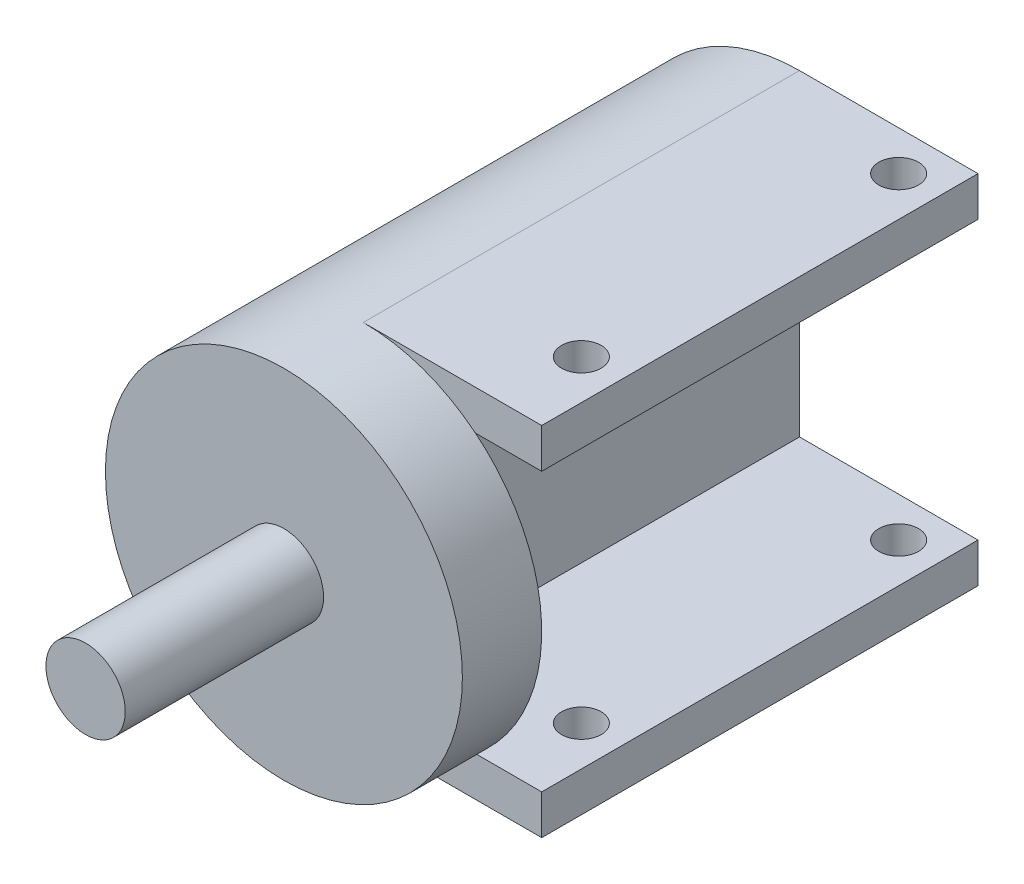
from build123d import *

# Parameters (mm, degrees)
SKETCH_1_R          = 22.5
EXTRUDE_1_DEPTH     = 65
SKETCH_2_R          = 5
EXTRUDE_2_DEPTH     = 25
SKETCH_3_W          = 22.5
SKETCH_3_H          = 55
EXTRUDE_3_DEPTH     = 5
SKETCH_4_W          = 22.5
SKETCH_4_H          = 55
EXTRUDE_4_DEPTH     = 5
CUT_EXTRUDE_1_DEPTH = 55
SKETCH_6_R          = 2.5
CUT_EXTRUDE_2_DEPTH = 60


with BuildPart() as part:
    # 草图1 → 凸台-拉伸1 (new body)
    with BuildSketch(Plane.XY):
        Circle(SKETCH_1_R)
    extrude(amount=EXTRUDE_1_DEPTH)

    # 草图2 → 凸台-拉伸2 (add)
    with BuildSketch(Plane.XY.offset(65)):
        Circle(SKETCH_2_R)
    extrude(amount=EXTRUDE_2_DEPTH)

    # 草图3 → 凸台-拉伸3 (add)
    with BuildSketch(Plane(origin=(0, 22.5, 0), x_dir=(-1, 0, 0), z_dir=(0, 1, 0))):
        with Locations((-11.25, 27.5)):
            Rectangle(SKETCH_3_W, SKETCH_3_H)
    extrude(amount=-EXTRUDE_3_DEPTH)

    # 草图4 → 凸台-拉伸4 (add)
    with BuildSketch(Plane(origin=(0, -22.5, 0), x_dir=(-1, 0, 0), z_dir=(0, 1, 0))):
        with Locations((-11.25, 27.5)):
            Rectangle(SKETCH_4_W, SKETCH_4_H)
    extrude(amount=EXTRUDE_4_DEPTH)

    # 草图5 → 切除-拉伸1 (cut)
    with BuildSketch(Plane(origin=(0, 0, 0), x_dir=(-1, 0, 0), z_dir=(0, 0, -1))):
        with BuildLine():
            Line((-14.142135624, -17.5), (0, -17.5))
            Line((0, -17.5), (0, 17.5))
            Line((0, 17.5), (-14.142135624, 17.5))
            ThreePointArc((-14.142135624, 17.5), (-22.5, 0), (-14.142135624, -17.5))
        make_face()
    extrude(amount=-CUT_EXTRUDE_1_DEPTH, mode=Mode.SUBTRACT)

    # 草图6 → 切除-拉伸2 (cut)
    with BuildSketch(Plane.XZ.offset(22.5)):
        with Locations(Location((17.5, 5, 0), (0, 0, 270))):
            Circle(SKETCH_6_R)
        with Locations(Location((17.5, 45, 0), (0, 0, 270))):
            Circle(SKETCH_6_R)
    extrude(amount=-CUT_EXTRUDE_2_DEPTH, mode=Mode.SUBTRACT)


solid = part.part
